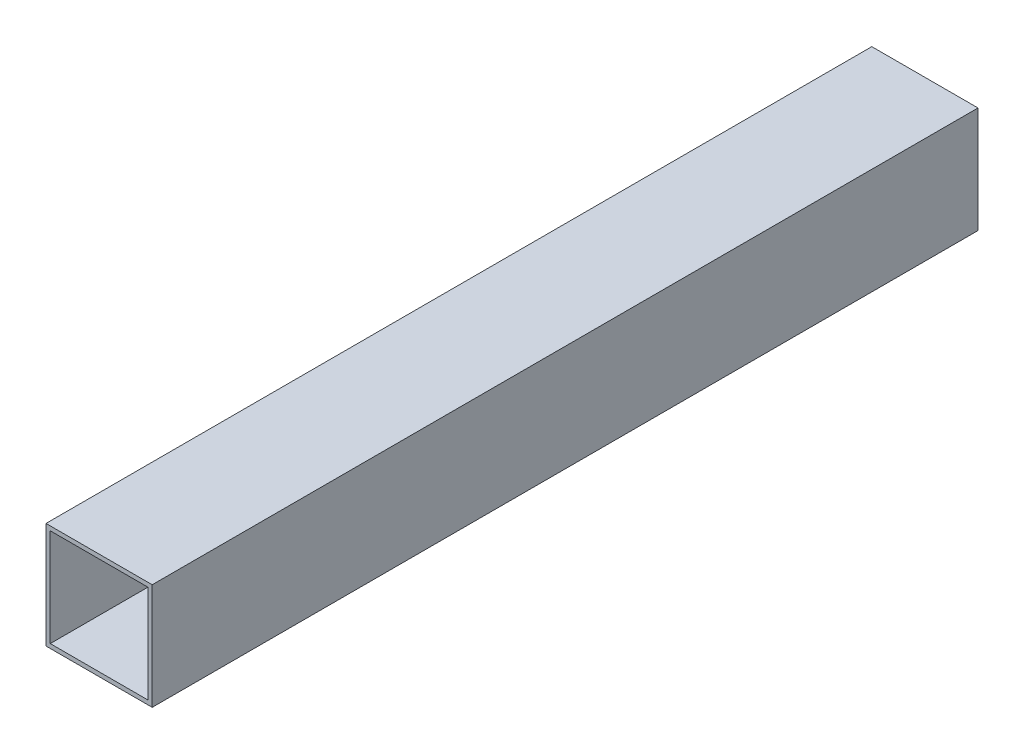
from build123d import *

# Parameters (mm, degrees)
SKETCH1_W           = 50
SKETCH1_H           = 50
SKETCH1_W_2         = 46
SKETCH1_H_2         = 46
BOSS_EXTRUDE1_DEPTH = 388.8


with BuildPart() as part:
    # Sketch1 → Boss-Extrude1 (new body)
    with BuildSketch(Plane.XY):
        Rectangle(SKETCH1_W, SKETCH1_H)
        Rectangle(SKETCH1_W_2, SKETCH1_H_2, mode=Mode.SUBTRACT)
    extrude(amount=BOSS_EXTRUDE1_DEPTH)


solid = part.part
